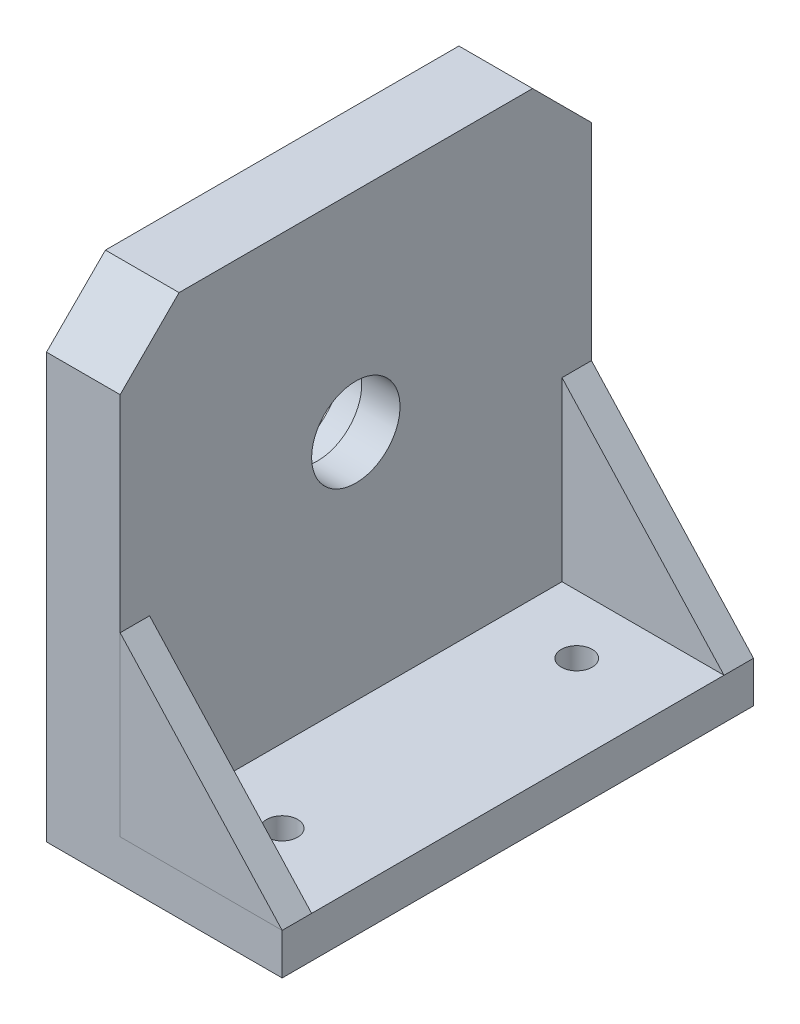
from build123d import *

# Parameters (mm, degrees)
SKETCH_1_W                         = 80
SKETCH_1_H                         = 160
EXTRUDE_1_DEPTH                    = 14
SKETCH_2_W                         = 25
SKETCH_2_H                         = 160
EXTRUDE_2_DEPTH                    = 150
EXTRUDE_3_DEPTH                    = 10
EXTRUDE_4_DEPTH                    = 10
SKETCH_5_R                         = 21
CUT_EXTRUDE_1_DEPTH                = 12
SKETCH_6_R                         = 15
CUT_EXTRUDE_2_DEPTH                = 195.730583114
HOLE_WIZARD_10_5_10_5_1_AT_2_COUNT = 2
HOLE_WIZARD_10_5_10_5_1_AT_2_PITCH = 100
CHAMFER_1_SIZE                     = 20


with BuildPart() as part:
    # 草图1 → 凸台-拉伸1 (new body)
    with BuildSketch(Plane(origin=(0, 0, 0), x_dir=(1, 0, 0), z_dir=(0, 1, 0))):
        Rectangle(SKETCH_1_W, SKETCH_1_H)
    extrude(amount=EXTRUDE_1_DEPTH)

    # 草图2 → 凸台-拉伸2 (add)
    with BuildSketch(Plane(origin=(0, 14, 0), x_dir=(1, 0, 0), z_dir=(0, 1, 0))):
        with Locations((-27.5, 0)):
            Rectangle(SKETCH_2_W, SKETCH_2_H)
    extrude(amount=EXTRUDE_2_DEPTH)

    # 草图5 → 切除-拉伸1 (cut)
    with BuildSketch(Plane.ZY.offset(40)):
        with Locations((0, 93)):
            Circle(SKETCH_5_R)
    extrude(amount=-CUT_EXTRUDE_1_DEPTH, mode=Mode.SUBTRACT)

    # 草图6 → 切除-拉伸2 (cut, through all)
    with BuildSketch(Plane.ZY.offset(28)):
        with Locations((0, 93)):
            Circle(SKETCH_6_R)
    extrude(amount=-CUT_EXTRUDE_2_DEPTH, mode=Mode.SUBTRACT)

    # 草图9 → Ø10.5 (10.5) 直径孔1 (revolve, cut)
    with BuildSketch(Plane(origin=(10, 14, -50), x_dir=(0, 0, 1), z_dir=(1, 0, 0))):
        Polygon((0, 0), (0, 18.15451825), (5.25, 15), (5.25, 0), align=None)
    hole_wizard_10_5_10_5_1 = revolve(axis=Axis((10, 20.35, -50), (0, -1, 0)), mode=Mode.SUBTRACT)

    # Ø10.5 (10.5) 直径孔1 at 2: Ø10.5 (10.5) 直径孔1 ×2
    with Locations(*[(0, 0, i * HOLE_WIZARD_10_5_10_5_1_AT_2_PITCH) for i in range(1, HOLE_WIZARD_10_5_10_5_1_AT_2_COUNT)]):
        add(hole_wizard_10_5_10_5_1, mode=Mode.SUBTRACT)

    # 倒角1
    chamfer_1_edges = [part.edges().sort_by_distance(p)[0] for p in [
        (-27.5, 164, 80),
        (-27.5, 164, -80),
    ]]
    chamfer(chamfer_1_edges, length=CHAMFER_1_SIZE)


with BuildPart() as body_2:
    # 草图3 → 凸台-拉伸3 (new body)
    with BuildSketch(Plane.XY.offset(80)):
        Polygon((-15, 74), (40, 14), (-15, 14), align=None)
    extrude(amount=-EXTRUDE_3_DEPTH)


with BuildPart() as body_3:
    # 草图4 → 凸台-拉伸4 (new body)
    with BuildSketch(Plane(origin=(0, 0, -80), x_dir=(-1, 0, 0), z_dir=(0, 0, -1))):
        Polygon((15, 14), (15, 74), (-40, 14), align=None)
    extrude(amount=-EXTRUDE_4_DEPTH)


solid = Compound([part.part, body_2.part, body_3.part])
